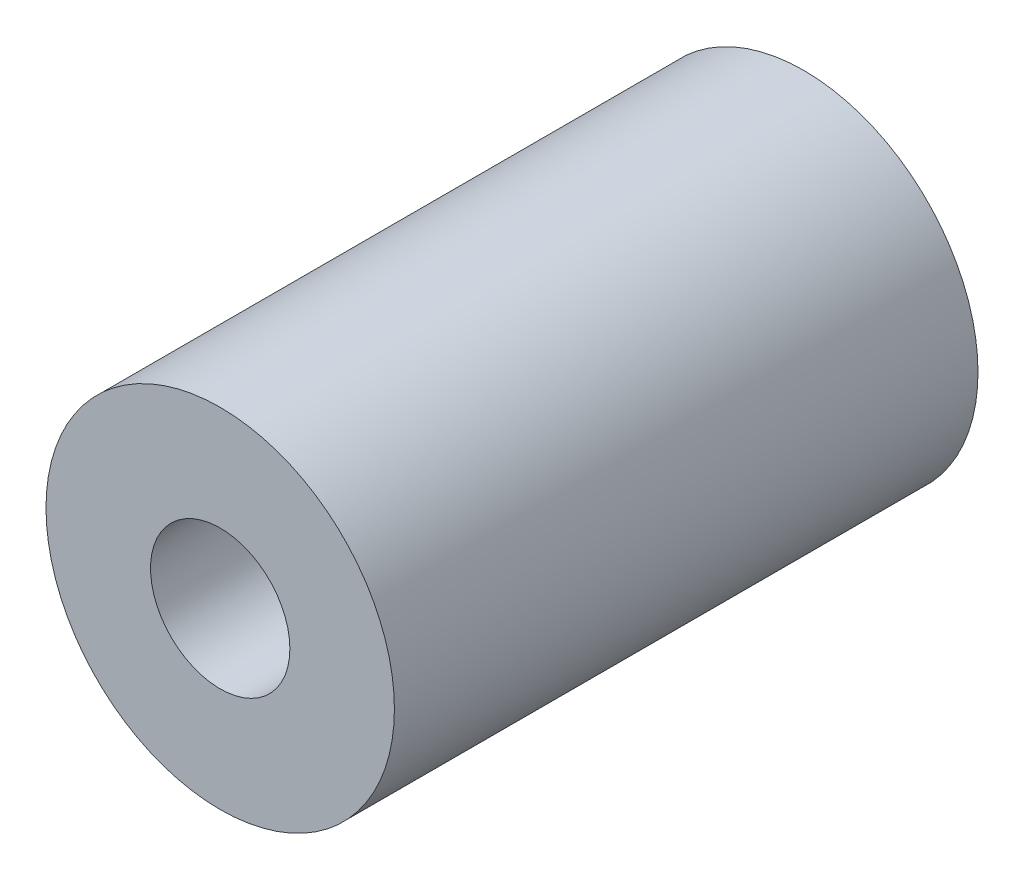
SolidWorks part; units mm, degrees
ref_plane "前视基准面" through (0, 0, 0) normal (0, 0, 1) x (1, 0, 0)
ref_plane "上视基准面" through (0, 0, 0) normal (0, 1, 0) x (1, 0, 0)
ref_plane "右视基准面" through (0, 0, 0) normal (1, 0, 0) x (0, 0, -1)
sketch "草图1" plane through (0, 0, 0) normal (0, 0, 1) x (1, 0, 0)
  circle A0 centre (0, 0) radius 20
  dimension "D1" = 40
extrude "凸台-拉伸1" add sketch "草图1" along normal blind 67
sketch "草图2" plane through (0, 0, 67) normal (0, 0, 1) x (1, 0, 0)
  circle A0 centre (0, 0) radius 8
  dimension "D1" = 16
extrude "切除-拉伸1" cut sketch "草图2" against normal blind 101
